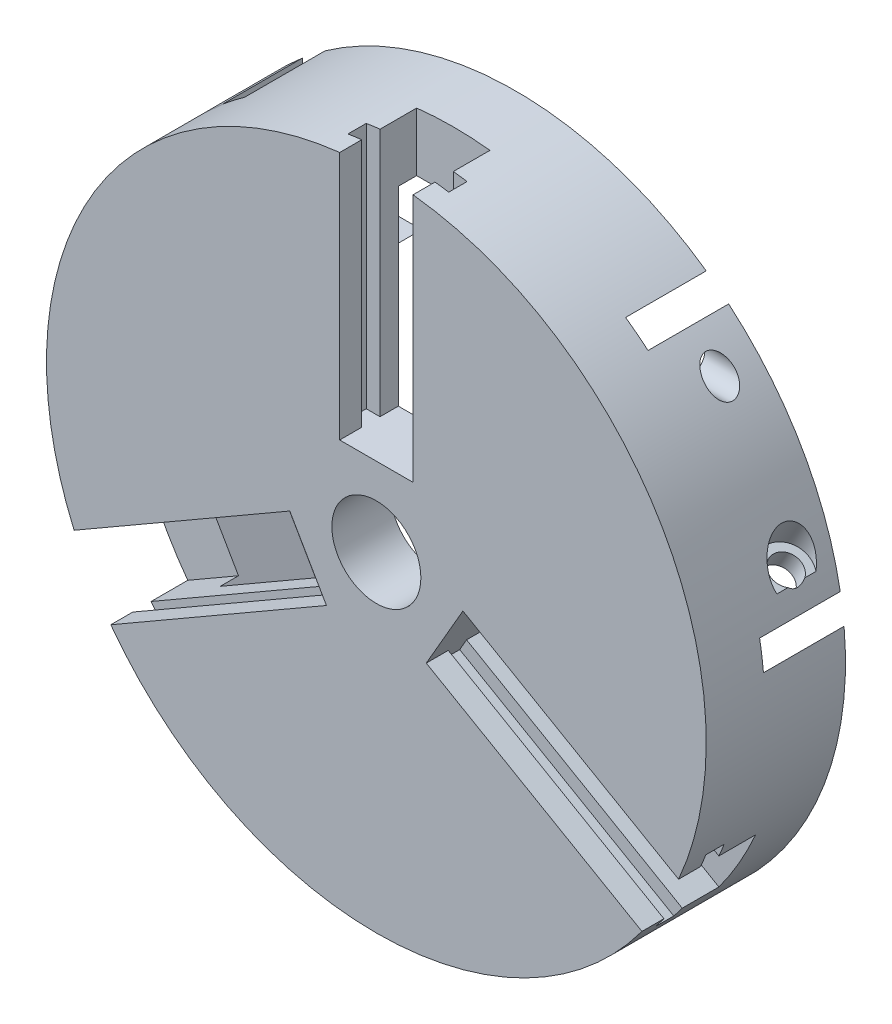
from build123d import *
from build123d.topology import SkipClean

# Parameters (mm, degrees)
SKETCH1_R                = 180
BOSS_EXTRUDE1_DEPTH      = 32
CUT_EXTRUDE1_DEPTH       = 40
CIRPATTERN1_COUNT        = 3
SKETCH3_W                = 10
SKETCH3_H                = 55
CUT_EXTRUDE2_DEPTH       = 160
CIRPATTERN2_COUNT        = 3
CUT_EXTRUDE3_DEPTH       = 1
BOSS_EXTRUDE2_DEPTH      = 44
BOSS_EXTRUDE2_DEPTH_BACK = 1
CIRPATTERN5_COUNT        = 3
CUT_EXTRUDE4_START       = -51
SKETCH6_R                = 8
CUT_EXTRUDE4_DEPTH       = 332
CIRPATTERN6_COUNT        = 3
SKETCH7_R                = 12.5
CUT_EXTRUDE5_DEPTH       = 30
CIRPATTERN7_COUNT        = 3
BOSS_EXTRUDE3_START      = 44
BOSS_EXTRUDE3_DEPTH      = 44
SKETCH11_W               = 10
SKETCH11_H               = 40
CUT_EXTRUDE8_DEPTH       = 160
SKETCH12_W               = 40
SKETCH12_H               = 10
CUT_EXTRUDE9_DEPTH       = 160
SKETCH13_W               = 10
SKETCH13_H               = 40
CUT_EXTRUDE10_DEPTH      = 160
SKETCH15_R               = 24.295855894
CUT_EXTRUDE12_DEPTH      = 40


with BuildPart() as part:
    # Sketch1 → Boss-Extrude1 (new body)
    with BuildSketch(Plane.XY):
        Circle(SKETCH1_R)
    extrude(amount=BOSS_EXTRUDE1_DEPTH)

    # Sketch2 → Cut-Extrude1 (cut)
    with BuildSketch(Plane.XY.offset(32)):
        with BuildLine():
            Line((20, 187.415434366), (20, 43))
            Line((20, 43), (-20, 43))
            Line((-20, 43), (-20, 187.415434366))
            ThreePointArc((-20, 187.415434366), (0, 188.479561328), (20, 187.415434366))
        make_face()
    cut_extrude1 = extrude(amount=-CUT_EXTRUDE1_DEPTH, mode=Mode.SUBTRACT)

    # CirPattern1: Cut-Extrude1 ×3 about axis
    cirpattern1_axis = Axis((0, 0, 0), (0, 0, 1))
    for i in range(1, CIRPATTERN1_COUNT):
        add(cut_extrude1.rotate(cirpattern1_axis, i * 360 / CIRPATTERN1_COUNT), mode=Mode.SUBTRACT)

    # Sketch3 → Cut-Extrude2 (cut)
    with BuildSketch(Plane(origin=(37.239092363, -21.5, 0), x_dir=(0, 0, -1), z_dir=(0.8660254037844365, -0.500000000000004, 0))):
        with Locations((-15, 0)):
            Rectangle(SKETCH3_W, SKETCH3_H)
    cut_extrude2 = extrude(amount=CUT_EXTRUDE2_DEPTH, mode=Mode.SUBTRACT)

    # CirPattern2: Cut-Extrude2 ×3 about axis
    cirpattern2_axis = Axis((0, 0, 0), (0, 0, 1))
    for i in range(1, CIRPATTERN2_COUNT):
        add(cut_extrude2.rotate(cirpattern2_axis, i * 360 / CIRPATTERN2_COUNT), mode=Mode.SUBTRACT)

    # Sketch4 → Cut-Extrude3 (cut)
    with BuildSketch(Plane(origin=(1185.054388592, -482.713178643, 0), x_dir=(1, 0, 0), z_dir=(0, 0, -1))):
        with BuildLine():
            Line((-1236.304388592, -571.480782531), (-1301.304388592, -571.480782531))
            Line((-1301.304388592, -571.480782531), (-1301.304388592, -620.139295157))
            ThreePointArc((-1301.304388592, -620.139295157), (-1340.938961274, -572.713178643), (-1362.193896637, -514.675573576))
            Line((-1362.193896637, -514.675573576), (-1320.054388592, -539.004829889))
            Line((-1320.054388592, -539.004829889), (-1287.554388592, -482.713178643))
            ThreePointArc((-1287.554388592, -482.713178643), (-1273.82199248, -533.963178643), (-1236.304388592, -571.480782531))
        make_face()
        with BuildLine():
            Line((-1133.804388592, -571.480782531), (-1068.804388592, -571.480782531))
            Line((-1068.804388592, -571.480782531), (-1068.804388592, -620.139295157))
            ThreePointArc((-1068.804388592, -620.139295157), (-1029.169815911, -572.713178643), (-1007.914880548, -514.675573576))
            Line((-1007.914880548, -514.675573576), (-1050.054388592, -539.004829889))
            Line((-1050.054388592, -539.004829889), (-1082.554388592, -482.713178643))
            ThreePointArc((-1082.554388592, -482.713178643), (-1096.286784705, -533.963178643), (-1133.804388592, -571.480782531))
        make_face()
        with BuildLine():
            Line((-1236.304388592, -393.945574755), (-1203.804388592, -337.653923509))
            Line((-1203.804388592, -337.653923509), (-1245.943896637, -313.324667197))
            ThreePointArc((-1245.943896637, -313.324667197), (-1185.054388592, -302.713178643), (-1124.164880548, -313.324667197))
            Line((-1124.164880548, -313.324667197), (-1166.304388592, -337.653923509))
            Line((-1166.304388592, -337.653923509), (-1133.804388592, -393.945574755))
            ThreePointArc((-1133.804388592, -393.945574755), (-1185.054388592, -380.213178643), (-1236.304388592, -393.945574755))
        make_face()
    extrude(amount=-CUT_EXTRUDE3_DEPTH, mode=Mode.SUBTRACT)



with BuildPart() as body_2:
    # Sketch5 → Boss-Extrude2 (new, two sides: drawn at the far end of the back side and taken through both)
    with BuildSketch(Plane(origin=(0, 0, 0), x_dir=(-1, 0, 0), z_dir=(0, 0, -1)).offset(-BOSS_EXTRUDE2_DEPTH_BACK)):
        with BuildLine():
            Line((-116.25, 137.426116514), (-116.25, 88.767603888))
            Line((-116.25, 88.767603888), (-51.25, 88.767603888))
            ThreePointArc((-51.25, 88.767603888), (-88.767603888, 51.25), (-102.5, 0))
            Line((-102.5, 0), (-135, 56.291651246))
            Line((-135, 56.291651246), (-177.139508044, 31.962394933))
            ThreePointArc((-177.139508044, 31.962394933), (-155.884572681, 90), (-116.25, 137.426116514))
        make_face()
    extrude(amount=BOSS_EXTRUDE2_DEPTH + BOSS_EXTRUDE2_DEPTH_BACK)


with BuildPart() as cirpattern5_1:
    # CirPattern5: pattern copy
    add(body_2.part.rotate(Axis((0, 0, 0), (0, 0, 1)), 1 * 360 / CIRPATTERN5_COUNT))


with BuildPart() as cirpattern5_2:
    # CirPattern5: pattern copy
    add(body_2.part.rotate(Axis((0, 0, 0), (0, 0, 1)), 2 * 360 / CIRPATTERN5_COUNT))


with BuildPart() as cut_extrude4_tool:
    # Sketch6 → Cut-Extrude4 (new body)
    with BuildSketch(Plane(origin=(58.125, 100.67545319, 0), x_dir=(0.8660254037857631, -0.49999999999770584, 0), z_dir=(-0.4999999999977059, -0.8660254037857632, 0)).offset(CUT_EXTRUDE4_START)):
        with Locations(Location((121.75, -23, 0), (0, 0, 180))):
            Circle(SKETCH6_R)
    cut_extrude4 = extrude(amount=CUT_EXTRUDE4_DEPTH)


with BuildPart() as body_2_1:
    add(body_2.part)

    # Cut-Extrude4: cut by cut_extrude4_tool
    add(cut_extrude4_tool.part, mode=Mode.SUBTRACT)


with BuildPart() as cirpattern5_2_1:
    add(cirpattern5_2.part)

    # Cut-Extrude4: cut by cut_extrude4_tool
    add(cut_extrude4_tool.part, mode=Mode.SUBTRACT)


with BuildPart() as cirpattern6_tool:
    # CirPattern6: Cut-Extrude4 ×3 about axis
    cirpattern6_axis = Axis((0, 0, 32), (0, 0, -1))
    for i in range(1, CIRPATTERN6_COUNT):
        add(cut_extrude4.rotate(cirpattern6_axis, i * 360 / CIRPATTERN6_COUNT))


with BuildPart() as body_2_2:
    add(body_2_1.part)

    # CirPattern6: cut by cirpattern6_tool
    add(cirpattern6_tool.part, mode=Mode.SUBTRACT)


with BuildPart() as cirpattern5_1_1:
    add(cirpattern5_1.part)

    # CirPattern6: cut by cirpattern6_tool
    add(cirpattern6_tool.part, mode=Mode.SUBTRACT)


with BuildPart() as cirpattern5_2_2:
    add(cirpattern5_2_1.part)

    # CirPattern6: cut by cirpattern6_tool
    add(cirpattern6_tool.part, mode=Mode.SUBTRACT)

    # Sketch7 → Cut-Extrude5 (cut)
    with BuildSketch(Plane(origin=(63.125, -109.335707228, 0), x_dir=(0.8660254037831165, 0.5000000000022902, 0), z_dir=(-0.5000000000022902, 0.8660254037831165, 0))):
        with Locations((-121.75, 23)):
            Circle(SKETCH7_R)
    cut_extrude5 = extrude(amount=-CUT_EXTRUDE5_DEPTH, mode=Mode.SUBTRACT)


with BuildPart() as cirpattern7_tool:
    # CirPattern7: Cut-Extrude5 ×3 about axis
    cirpattern7_axis = Axis((0, 0, 0), (0, 0, 1))
    for i in range(1, CIRPATTERN7_COUNT):
        add(cut_extrude5.rotate(cirpattern7_axis, i * 360 / CIRPATTERN7_COUNT))


with BuildPart() as body_2_3:
    add(body_2_2.part)

    # CirPattern7: cut by cirpattern7_tool
    add(cirpattern7_tool.part, mode=Mode.SUBTRACT)


with BuildPart() as cirpattern5_1_2:
    add(cirpattern5_1_1.part)

    # CirPattern7: cut by cirpattern7_tool
    add(cirpattern7_tool.part, mode=Mode.SUBTRACT)


with BuildPart() as part_1:
    with SkipClean():  # the faces are left unmerged after this step: merging them gives an invalid solid
        add(part.part)

        add(body_2_3.part)  # Boss-Extrude3 merges body 2
        # Sketch10 → Boss-Extrude3 (add)
        with BuildSketch(Plane(origin=(0, 0, 0), x_dir=(-1, 0, 0), z_dir=(0, 0, -1)).offset(BOSS_EXTRUDE3_START)):
            with BuildLine():
                Line((-179.232071429, 16.609171305), (-75.232071429, -163.524112682))
                ThreePointArc((-75.232071429, -163.524112682), (-155.884572681, -90), (-179.232071429, 16.609171305))
            make_face()
            with BuildLine():
                Line((104, 146.914941378), (-104, 146.914941378))
                ThreePointArc((-104, 146.914941378), (0, 180), (104, 146.914941378))
            make_face()
            with BuildLine():
                Line((75.232071429, -163.524112682), (179.232071429, 16.609171305))
                ThreePointArc((179.232071429, 16.609171305), (155.884572682, -90), (75.232071429, -163.524112682))
            make_face()
        extrude(amount=-BOSS_EXTRUDE3_DEPTH)

    # Sketch11 → Cut-Extrude8 (cut)
    with BuildSketch(Plane(origin=(-37.239092363, -21.5, 0), x_dir=(0, 0, 1), z_dir=(-0.8660254037844431, -0.4999999999999923, 0))):
        with Locations((-5, 0)):
            Rectangle(SKETCH11_W, SKETCH11_H)
    extrude(amount=CUT_EXTRUDE8_DEPTH, mode=Mode.SUBTRACT)

    # Sketch12 → Cut-Extrude9 (cut)
    with BuildSketch(Plane(origin=(0, 43, 0), x_dir=(1, 0, 0), z_dir=(0, 1, 0))):
        with Locations((0, 5)):
            Rectangle(SKETCH12_W, SKETCH12_H)
    extrude(amount=CUT_EXTRUDE9_DEPTH, mode=Mode.SUBTRACT)

    # Sketch13 → Cut-Extrude10 (cut)
    with BuildSketch(Plane(origin=(37.239092363, -21.5, 0), x_dir=(0, 0, -1), z_dir=(0.8660254037844365, -0.500000000000004, 0))):
        with Locations((5, 0)):
            Rectangle(SKETCH13_W, SKETCH13_H)
    extrude(amount=CUT_EXTRUDE10_DEPTH, mode=Mode.SUBTRACT)

    # Sketch15 → Cut-Extrude12 (cut)
    with BuildSketch(Plane.XY.offset(32)):
        Circle(SKETCH15_R)
    extrude(amount=-CUT_EXTRUDE12_DEPTH, mode=Mode.SUBTRACT)


solid = Compound([cirpattern5_2_2.part, cirpattern5_1_2.part, part_1.part])
